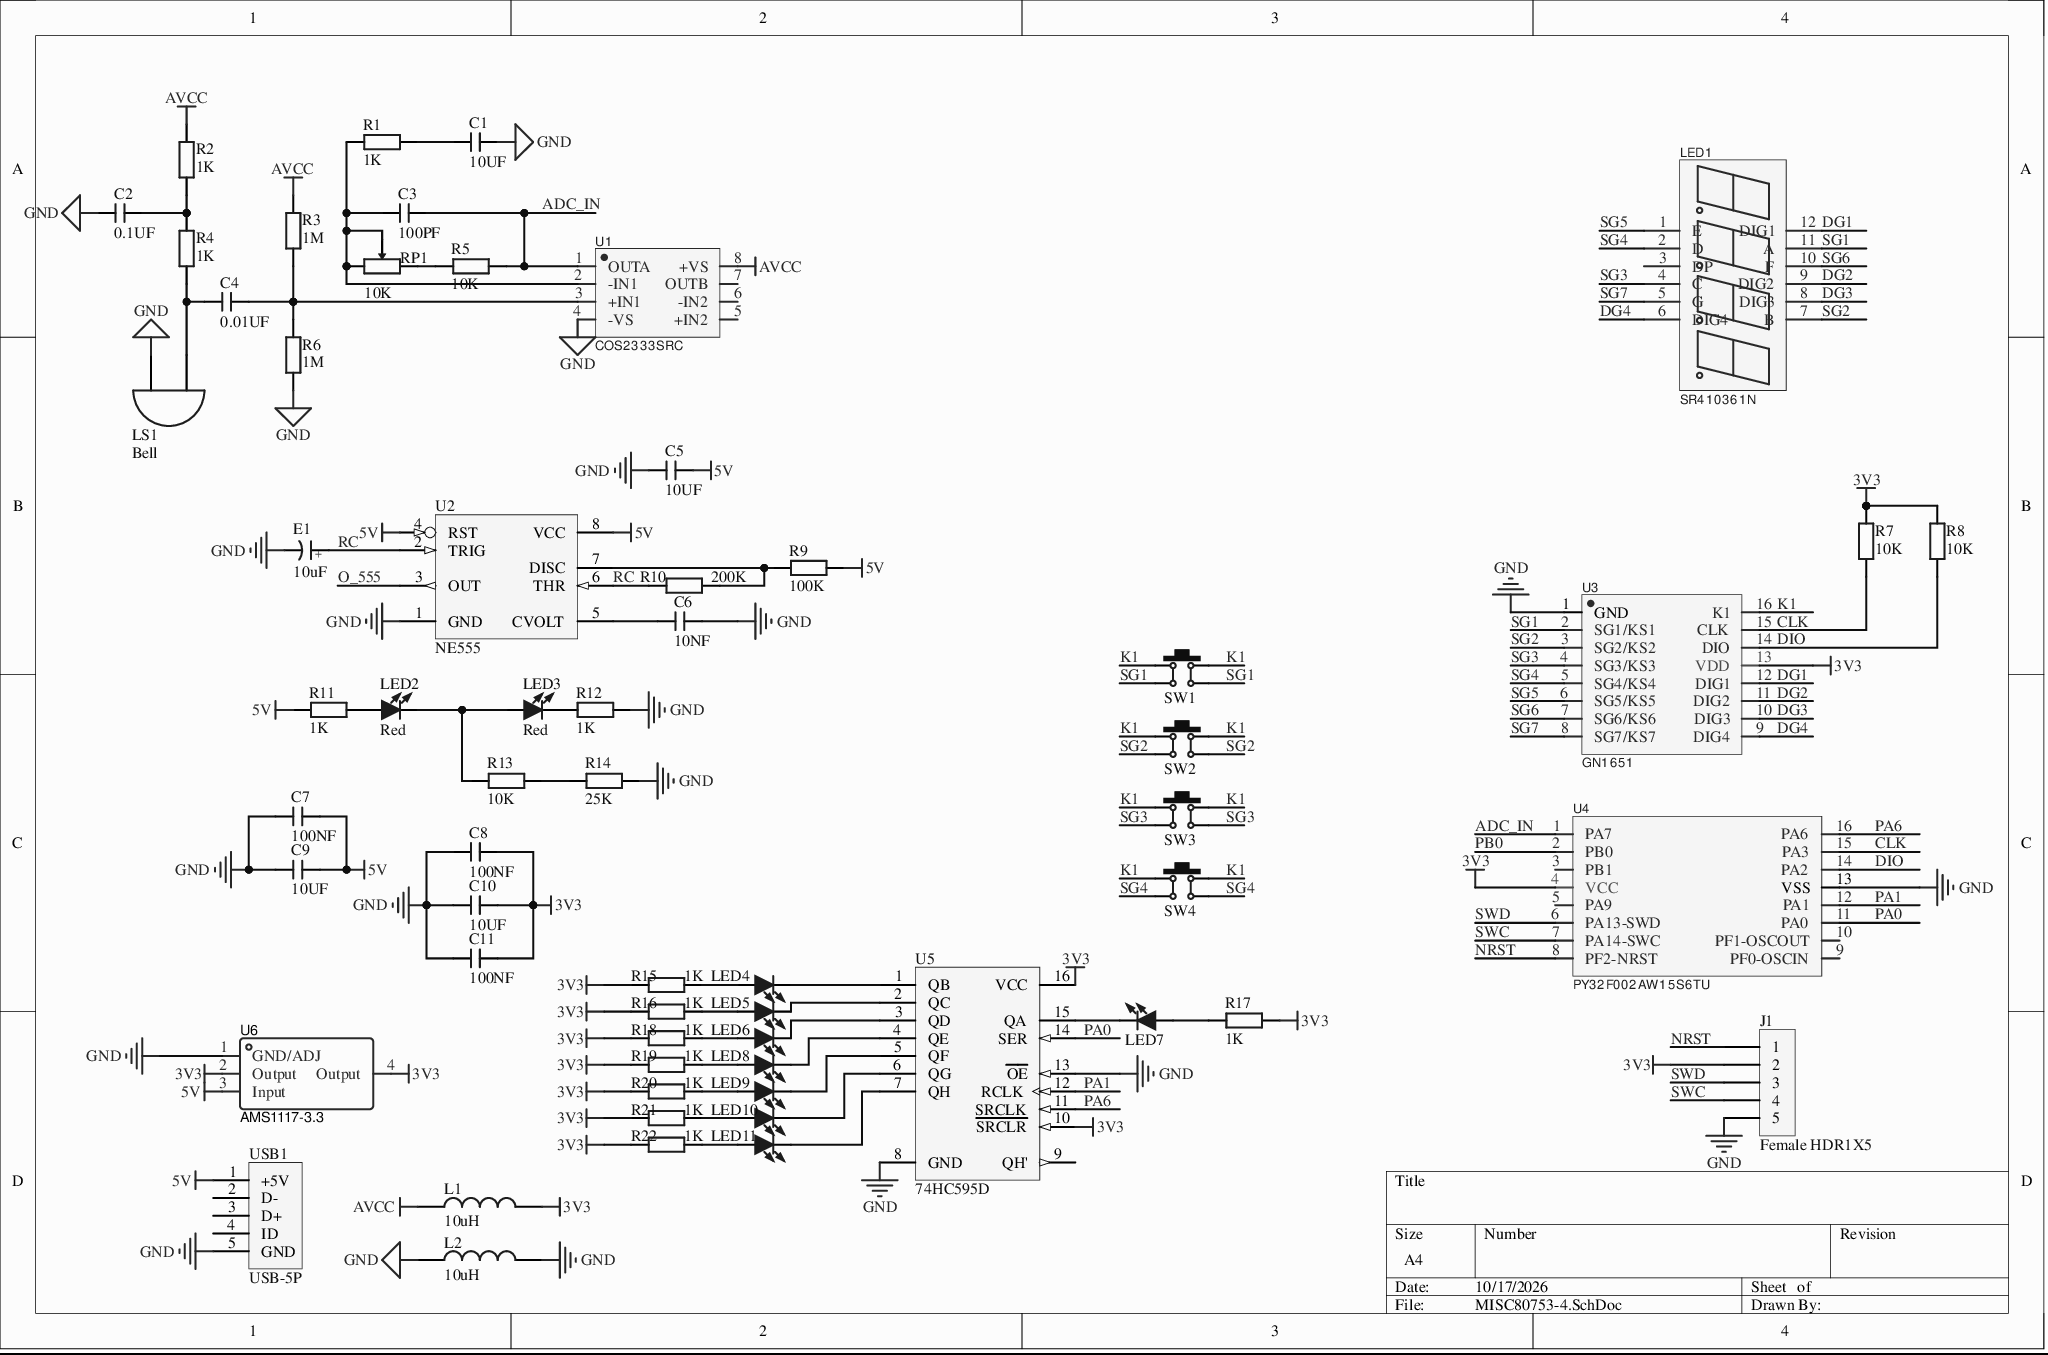
[diagram p0: MISC80753-4.SchDoc]
# Altium project MISC80753-7.PrjPcb
1 sheet, 61 parts. Net scope: global (net labels, ports and power ports of the same name join across sheets).
Board file: MISC80753.PcbDoc

## Sheet MISC80753-4.SchDoc
size A4

### Parts
C1  10UF  [C 0805_L]
C2  0.1UF  [C 0805_L]
C3  100PF  [C 0805_L]
C4  0.01UF  [C 0805_L]
C5  10UF  [C 0805_L]
C6  10NF  [C 0805_L]
C7  100NF  [C 0805_L]
C8  100NF  [C 0805_L]
C9  10UF  [C 0805_L]
C10  10UF  [C 0805_L]
C11  100NF  [C 0805_L]
E1  10uF  [CM A(3*5.4)]
J1  Female HDR1X5  [Fe-HDR1X5/2.54-S]
L1  10uH  [L 0805]
L2  10uH  [L 0805]
LED1  SR410361N  [LED-SEG-TH_12P-L30.0-W14.0-P2.54-S10.26-BL]
LED2  Red  [LED 0805G]
LED3  Red  [LED 0805G]
LED4  Red  [LED 0805G]  (value not drawn)
LED5  Red  [LED 0805G]  (value not drawn)
LED6  Red  [LED 0805G]  (value not drawn)
LED7  Red  [LED 0805G]  (value not drawn)
LED8  Red  [LED 0805G]  (value not drawn)
LED9  Red  [LED 0805G]  (value not drawn)
LED10  Red  [LED 0805G]  (value not drawn)
LED11  Red  [LED 0805G]  (value not drawn)
LS1  Bell  [PIN2]
R1  1K  [R 0805_L]
R2  1K  [R 0805_L]
R3  1M  [R 0805_L]
R4  1K  [R 0805_L]
R5  10K  [R 0805_L]
R6  1M  [R 0805_L]
R7  10K  [R 0805_L]
R8  10K  [R 0805_L]
R9  100K  [R 0805_L]
R10  200K  [R 0805_L]
R11  1K  [R 0805_L]
R12  1K  [R 0805_L]
R13  10K  [R 0805_L]
R14  25K  [R 0805_L]
R15  1K  [R 0805_L]
R16  1K  [R 0805_L]
R17  1K  [R 0805_L]
R18  1K  [R 0805_L]
R19  1K  [R 0805_L]
R20  1K  [R 0805_L]
R21  1K  [R 0805_L]
R22  1K  [R 0805_L]
RP1  10K  [3296W]
SW1  6x6x5  [四脚轻触开关]  (value not drawn)
SW2  6x6x5  [四脚轻触开关]  (value not drawn)
SW3  6x6x5  [四脚轻触开关]  (value not drawn)
SW4  6x6x5  [四脚轻触开关]  (value not drawn)
U1  COS2333SRC  [SOP-8_L4.9-W3.9-P1.27-LS6.0-BL]
U2  NE555  [SOP8]
U3  GN1651  [SOP-16_L9.9-W3.9-P1.27-LS6.1-BL]
U4  PY32F002AW15S6TU  [SOP-16_L9.9-W3.9-P1.27-LS6.0-BL]
U5  74HC595D  [SOP16]
U6  AMS1117-3.3  [AMS1117-3.3]
USB1  USB-5P  [USB-MICRO_A]

### Nets
3V3: C8.2 C10.2 C11.2 J1.2 L1.2 R7.2 R8.2 R15.1 R16.1 R17.1 R18.1 R19.1 R20.1 R21.1 R22.1 U3.13(VDD) U4.4(VCC) U5.10(~{SRCLR}) U5.16(VCC) U6.2(Output) U6.4(Output)
5V: C5.2 C7.2 C9.2 R9.2 R11.1 U2.4(RST) U2.8(VCC) U6.3(Input) USB1.1(+5V)
AVCC: L1.1 R2.2 R3.2 U1.8(+VS)
GND: C1.2 C2.1 C5.1 C6.2 C7.1 C8.1 C9.1 C10.1 C11.1 E1.2(K) J1.5 L2.1 L2.2 LS1.2(B) R6.2 R12.2 R14.2 U1.4(-VS) U2.1(GND) U3.1(GND) U4.13(VSS) U5.8(GND) U5.13(~{OE}) U6.1(GND/ADJ) USB1.5(GND)
ADC_IN: C3.2 R5.2 U1.1(OUTA) U4.1(PA7)
CLK: R7.1 U3.15(CLK) U4.15(PA3)
DG1: LED1.12(DIG1) U3.12(DIG1)
DG2: LED1.9(DIG2) U3.11(DIG2)
DG3: LED1.8(DIG3) U3.10(DIG3)
DG4: LED1.6(DIG4) U3.9(DIG4)
DIO: R8.1 U3.14(DIO) U4.14(PA2)
K1: SW1.1 SW1.2 SW2.1 SW2.2 SW3.1 SW3.2 SW4.1 SW4.2 U3.16(K1)
NRST: J1.1 U4.8(PF2-NRST)
O_555: U2.3(OUT)
PA0: U4.11(PA0) U5.14(SER)
PA1: U4.12(PA1) U5.12(RCLK)
PA6: U4.16(PA6) U5.11(SRCLK)
PB0: U4.2(PB0)
RC: E1.1(A) R10.1 U2.2(TRIG) U2.6(THR)
SG1: LED1.11(A) SW1.3 SW1.4 U3.2(SG1/KS1)
SG2: LED1.7(B) SW2.3 SW2.4 U3.3(SG2/KS2)
SG3: LED1.4(C) SW3.3 SW3.4 U3.4(SG3/KS3)
SG4: LED1.2(D) SW4.3 SW4.4 U3.5(SG4/KS4)
SG5: LED1.1(E) U3.6(SG5/KS5)
SG6: LED1.10(F) U3.7(SG6/KS6)
SG7: LED1.5(G) U3.8(SG7/KS7)
SWC: J1.4 U4.7(PA14-SWC)
SWD: J1.3 U4.6(PA13-SWD)
NetC1_1: C1.1 R1.2
NetC2_2: C2.2 R2.1 R4.2
NetC3_1: C3.1 R1.1 RP1.1 RP1.2 U1.2(-IN1)
NetC4_1: C4.1 LS1.1(A) R4.1
NetC4_2: C4.2 R3.1 R6.1 U1.3(+IN1)
NetC6_1: C6.1 U2.5(CVOLT)
NetLED2_1: LED2.1(A) R11.2
NetLED2_2: LED2.2(K) LED3.1(A) R13.1
NetLED3_2: LED3.2(K) R12.1
NetLED4_1: LED4.1(A) R15.2
NetLED4_2: LED4.2(K) U5.1(QB)
NetLED5_1: LED5.1(A) R16.2
NetLED5_2: LED5.2(K) U5.2(QC)
NetLED6_1: LED6.1(A) R18.2
NetLED6_2: LED6.2(K) U5.3(QD)
NetLED7_1: LED7.1(A) R17.2
NetLED7_2: LED7.2(K) U5.15(QA)
NetLED8_1: LED8.1(A) R19.2
NetLED8_2: LED8.2(K) U5.4(QE)
NetLED9_1: LED9.1(A) R20.2
NetLED9_2: LED9.2(K) U5.5(QF)
NetLED10_1: LED10.1(A) R21.2
NetLED10_2: LED10.2(K) U5.6(QG)
NetLED11_1: LED11.1(A) R22.2
NetLED11_2: LED11.2(K) U5.7(QH)
NetR5_1: R5.1 RP1.3
NetR9_1: R9.1 R10.2 U2.7(DISC)
NetR13_2: R13.2 R14.1

Not connected (* = marked no-connect by the designer): LED1 3(DP); U1 5(+IN2) 6(-IN2) 7(OUTB); U4 3(PB1) 5(PA9) 9(PF0-OSCIN) 10(PF1-OSCOUT); U5 9(QH'); USB1 2(D-) 3(D+) 4(ID)

### Library data of the parts
C1-C11 = C: Chip capacitor; BOM名称: Non-polar chip capacitor
E1 = CE_SMD: Chip electrolytic capacitor; BOM名称: Chip electrolytic capacitor
L1 L2 = L: Low-power chip inductor; BOM名称: Low-power chip inductor
LED2-LED11 = LED-SMD: Chip LED; BOM名称: Chip LED
LS1 = Bell: Electrical Bell; Published: 24-Mar-1999; LatestRevisionDate: 17-Jul-2002; LatestRevisionNote: Re-released for DXP Platform.; PackageReference: PIN2; Publisher: Altium Limited
R1-R22 = R: Chip resistor; BOM名称: Chip resistor
RP1 = RP: Single-gang potentiometer; BOM名称: Through-hole potentiometer
SW1-SW4 = TSW DIP-6x6: Through-hole 6x6 tactile switch; BOM名称: Through-hole 6x6 tactile switch
U2 = NE555D: General-Purpose Single Bipolar Timer; Package Information: Latest Revision: Jul-1998; Code - JEDEC: MS-012-AA; Code - IPC: SO8; Published: 24-Aug-2001; Revision: 17-Jul-2002: Re-released for DXP Platform.; Datasheet: Latest Revision: Jul-1998; Package Reference: SO8; Publisher: Altium Limited
U5 = SN74HC595D: 8-Bit Shift Register with 3-State Output Registers; Package Information: Latest Revision: Jan-1998; Published: 8-Jun-2000; Revision: 17-Jul-2002: Re-released for DXP Platform.; Datasheet: Latest Revision: May-1997; Package Reference: D016; Publisher: Altium Limited
U6 = AMS1117-3.3: Manufacturer: KEXIN; Contributor: LCSC; SMT Type: Extend; Supplier: LCSC; Supplier Part: C369933; Manufacturer Part: AMS1117-3.3; JLCPCB SMD: Yes; spicePre: U; spiceSymbolName: AMS1117-3.3_C369933
USB1 = USB-5P: Micro USB female socket; BOM名称: Micro USB female socket